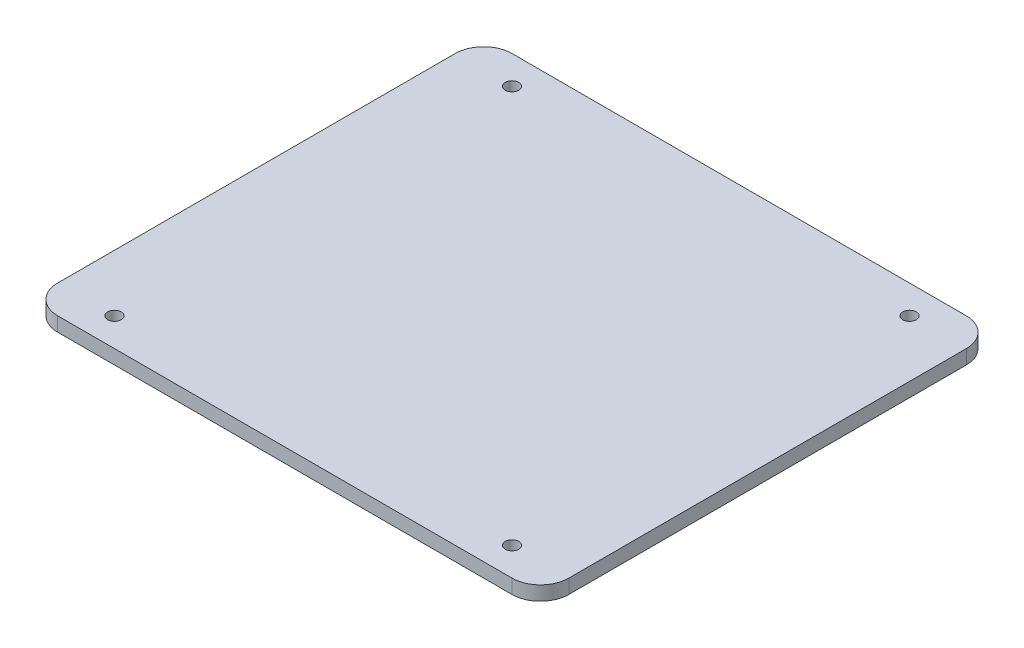
from build123d import *

# Parameters (mm, degrees)
SKETCH1_W            = 180
SKETCH1_H            = 160
BOSS_EXTRUDE1_DEPTH  = 2.5
M4_CLEARANCE_HOLE1_D = 4.8
FILLET1_R            = 10


with BuildPart() as part:
    # Sketch1 → Boss-Extrude1 (new, symmetric)
    with BuildSketch(Plane(origin=(0, 0, 0), x_dir=(1, 0, 0), z_dir=(0, 1, 0))):
        Rectangle(SKETCH1_W, SKETCH1_H)
    extrude(amount=BOSS_EXTRUDE1_DEPTH, both=True)

    # M4 Clearance Hole1 (through all)
    with Locations(Plane(origin=(-70, 2.5, -70), x_dir=(0, 0, 1), z_dir=(0, 1, 0))):
        with Locations((0, 0), (0, 140), (140, 140), (140, 0)):
            Hole(M4_CLEARANCE_HOLE1_D / 2)

    # Fillet1
    fillet1_edges = [part.edges().sort_by_distance(p)[0] for p in [
        (90, 0, 80),
        (-90, 0, 80),
        (-90, 0, -80),
        (90, 0, -80),
    ]]
    fillet(fillet1_edges, radius=FILLET1_R)


solid = part.part
